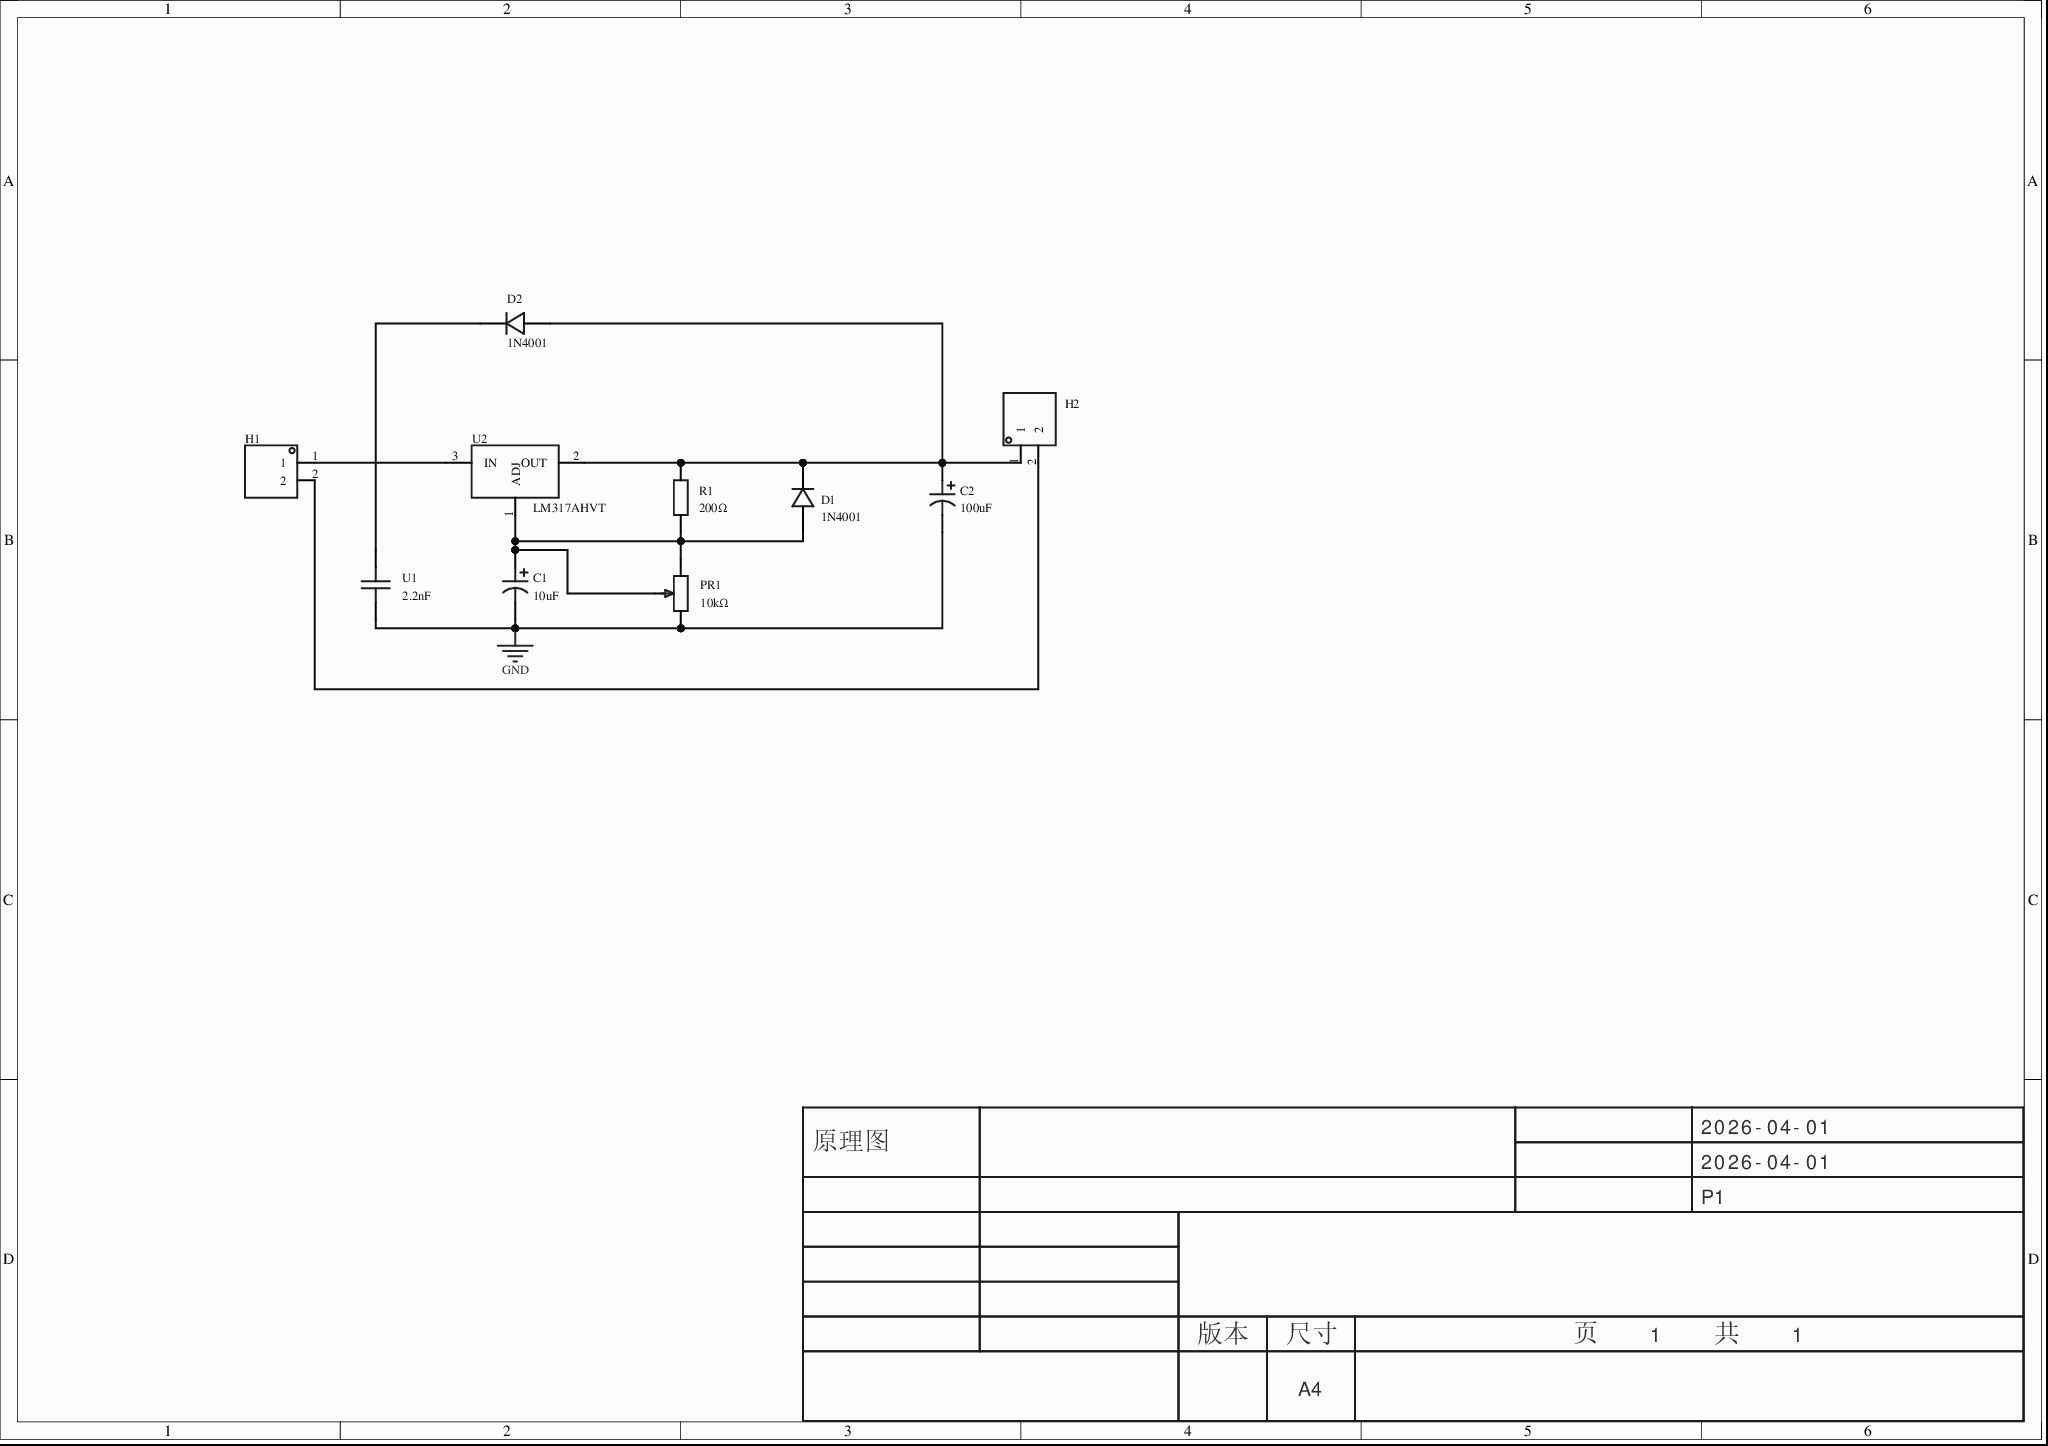
[diagram p0: MISC49891-3.schdoc]
# Altium project MISC49891-2.PrjPcb
1 sheet, 10 parts. Net scope: global (net labels, ports and power ports of the same name join across sheets).
Board file: MISC49891.pcbdoc

## Sheet MISC49891-3.schdoc
size 297 x 209 mm; Version: V1.0; @Project Name: MISC49891; @Update Date: 2026-04-01; @Create Date: 2026-04-01; @Board Name: MISC49891; @Create Time: 07:53:35; @Page Count: 1; @Page No: 1; @Schematic Name: MISC49891; @Update Time: 07:53:35; Size: A4

### Parts
C1  10uF  [CAP-TH_BD5.0-P2.00-D0.8-FD-10UF50VC110GL]
C2  100uF  [CAP-TH_BD8.0-P3.50-D0.6-FD_1]
D1  1N4001  [DO-41_BD2.4-L4.7-P8.70-D0.8-RD]
D2  1N4001  [DO-41_BD2.4-L4.7-P8.70-D0.8-RD]
H1  (no value)  [HDR-TH_2P-P2.54-V-M-1]
H2  (no value)  [HDR-TH_2P-P2.54-V-M-1]
PR1  10kΩ  [R_3296]
R1  200Ω  [Res_1/8W]
U1  2.2nF  [CAP-TH_L5.0-W2.5-P5.00-D1.0]
U2  LM317AHVT  [TO-220-3_L10.0-W4.5-P2.54-L]

### Nets
GND: C1.2 C2.2 PR1.3 U1.2
NetC1_1: C1.1 D1.2(A) PR1.1 PR1.2 R1.1 U2.1(ADJ)
NetC2_1: C2.1 D1.1(K) D2.2(A) H2.1 R1.2 U2.2(OUT)
NetD2_1: D2.1(K) U1.1
NetH1_1: H1.1 U2.3(IN)
NetH1_2: H1.2 H2.2

### Notes on the sheet
- 2026-04-01
- 原理图
- P1
- 版本
- 尺寸
- A4
- 页    1    共    1

### Library data of the parts
C1 = 10UF50VC110GL: 容值:10uF;精度:±20%;额定电压:50V;纹波电流:120mA@100KHz;等效串联电阻(ESR):1.6Ω;; Manufacturer: Econd(米朗电子); AddInBom: yes; Tolerance: ±20%; Voltage Rating: 50V; Equivalent Series Resistance(ESR): 1.6Ω; Pin Spacing: 2mm; Lifetime: 5000hrs@105℃; Symbol: 10UF50VC110GL; Device: 10UF50VC110GL; LCSC Part Name: 10uF ±20% 50V; SupplierPart: C46867109; ManufacturerPart: 10UF50VC110GL; Supplier Footprint: 插件,D5xL11mm; JLCPCB Part Class: Extended Part; Datasheet: https://item.szlcsc.com/datasheet/10UF50VC110GL/49031974.html; Supplier: LCSC; ConvertToPcb: yes; FootprintName: CAP-TH_BD5.0-P2.00-D0.8-FD-10UF50VC110GL; Value: 10uF; Ripple Current: 120mA@100KHz; Diameter: 5mm; Height - Seated (Max): 11mm; Operating Temperature: -40℃~+105℃
C2 = 100uF: Symbol: 100UF_C9900016884; AddInBom: yes; ModelId: 5fc21599cab34df2ad7753b19b2f52860819f05c4eef4c71ace90d822a990e87; ModelTransform: 315.365,314.914,0,0,0,0,0,0,-196.85; Device: 100uF; LCSC Part Name: 100uF; SupplierPart: C9900016884; ManufacturerPart: 100uF; Supplier Footprint: CAP-TH_BD8.0-P3.50-D1.0-FD; JLCPCB Part Class: Extended Part; Supplier: LCSC; ConvertToPcb: yes; FootprintName: CAP-TH_BD8.0-P3.50-D0.6-FD_1; ModelName: CAP-TH_BD8.0-P3.50-D0.6-FD_1
D1 D2 = 1N4001E-E3/73: Manufacturer: VISHAY(威世); AddInBom: yes; ModelId: 6de1e9b71a0d4751b4e9df530304c1a30819f05c4eef4c71ace90d822a990e87; ModelName: DO-41_D2.4-L4.7-P8.70; ModelTransform: 374.015,94.428,0,0,0,0,0,0,-137.795; Symbol: 1N4001E-E3/73; Device: 1N4001E-E3/73; Manufacturer Part: 1N4001; LCSC Part Name: 1N4001E-E3/73; SupplierPart: C26137025; Supplier Footprint: -; Datasheet: https://atta.szlcsc.com/upload/public/pdf/source/20241111/0150693623A5BDBCEC36A998B7AC180D.pdf; Supplier: LCSC; ConvertToPcb: yes; FootprintName: DO-41_BD2.4-L4.7-P8.70-D0.8-RD
H1 H2 = HDR-M_2.54_1x2P: Symbol: 210S-1*2P L=11.6MMGold-plated black; ConvertToPcb: yes; ModelId: 79b2e9f2d70a4d68a1b7098f27c6d4c50819f05c4eef4c71ace90d822a990e87; ModelName: HDR-M-2.54_1x2; ModelTransform: 200,100,0,0,0,0,0,0,-118.11; Device: HDR-M_2.54_1x2P; AddInBom: yes; SupplierPart: C124375; Supplier Footprint: 插件; FootprintName: HDR-TH_2P-P2.54-V-M-1
PR1 = R_3296: ConvertToPcb: yes; ModelId: b182808559bb43bda9e7de64b64134cb0819f05c4eef4c71ace90d822a990e87; ModelName: 3296W; ModelTransform: 373.98,188.96,590.49,180,0,0,0,0,-140; Symbol: R_3296; Device: R_3296; AddInBom: yes; Supplier Footprint: 直插; FootprintName: R_3296; Value: 10kΩ
R1 = Res_AXIAL-1/8W: Symbol: 电阻; ConvertToPcb: yes; ModelId: b2b5ae7ae4c642178fe0039925c86a3f0819f05c4eef4c71ace90d822a990e87; ModelName: RES-TH_BD1.8-L3.2-P7.20-D0.4; ModelTransform: 282.86,66.88,253.09,0,0,0,0,0,-191; Device: Res_AXIAL-1/8W; Value: 200Ω; AddInBom: yes; Supplier Footprint: 轴向引线; FootprintName: Res_1/8W
U1 = 100nF: Symbol: 100NF_C9900015256; AddInBom: yes; ModelId: 08e3d7481fc7486bb1b263873f51e1e10819f05c4eef4c71ace90d822a990e87; ModelName: CAP-TH_BD5.0-W2.5-P5.08; ModelTransform: 224.652,98.425,0,0,0,0,-0.005,0,-137.795; Device: 100nF; Manufacturer Part: 2.2nF; LCSC Part Name: 100nF; SupplierPart: C9900015256; Supplier Footprint: CAP-TH_L5.0-W2.5-P5.00-D1.0; JLCPCB Part Class: Extended Part; Supplier: LCSC; ConvertToPcb: yes; FootprintName: CAP-TH_L5.0-W2.5-P5.00-D1.0
U2 = LM317AHVT: 输出类型:可调;工作电压:-;输出电压:1.2V~57V;输出电流:1.5A;电源纹波抑制比(PSRR):75dB@(120Hz);输出极性:正极;; Manufacturer: onsemi(安森美); AddInBom: yes; ModelId: b3c9e38e4428458f8b925050989b538f0819f05c4eef4c71ace90d822a990e87; ModelTransform: 401.574,178.58232,0,0,0,0,0,25.59,-196.85; Output Type: 可调; Output Current: 1.5A; Output Configuration: 正极; Number of Outputs: 1; Symbol: LM317AHVT; Device: LM317AHVT; LCSC Part Name: 1.2V~57V 1.5A; SupplierPart: C111074; ManufacturerPart: LM317AHVT; Supplier Footprint: TO-220-3L; JLCPCB Part Class: Extended Part; Datasheet: https://item.szlcsc.com/datasheet/LM317AHVT/112300.html; Supplier: LCSC; ConvertToPcb: yes; FootprintName: TO-220-3_L10.0-W4.5-P2.54-L; ModelName: TO-220-3_L10.0-W4.5-P2.54-L; Voltage - Supply: -; Output Voltage: 1.2V~57V; Power Supply Rejection Ratio (PSRR): 75dB@(120Hz); Voltage Dropout: -; standby current: -; Noise: -; Operating Temperature: -40℃~+125℃@(Tj)